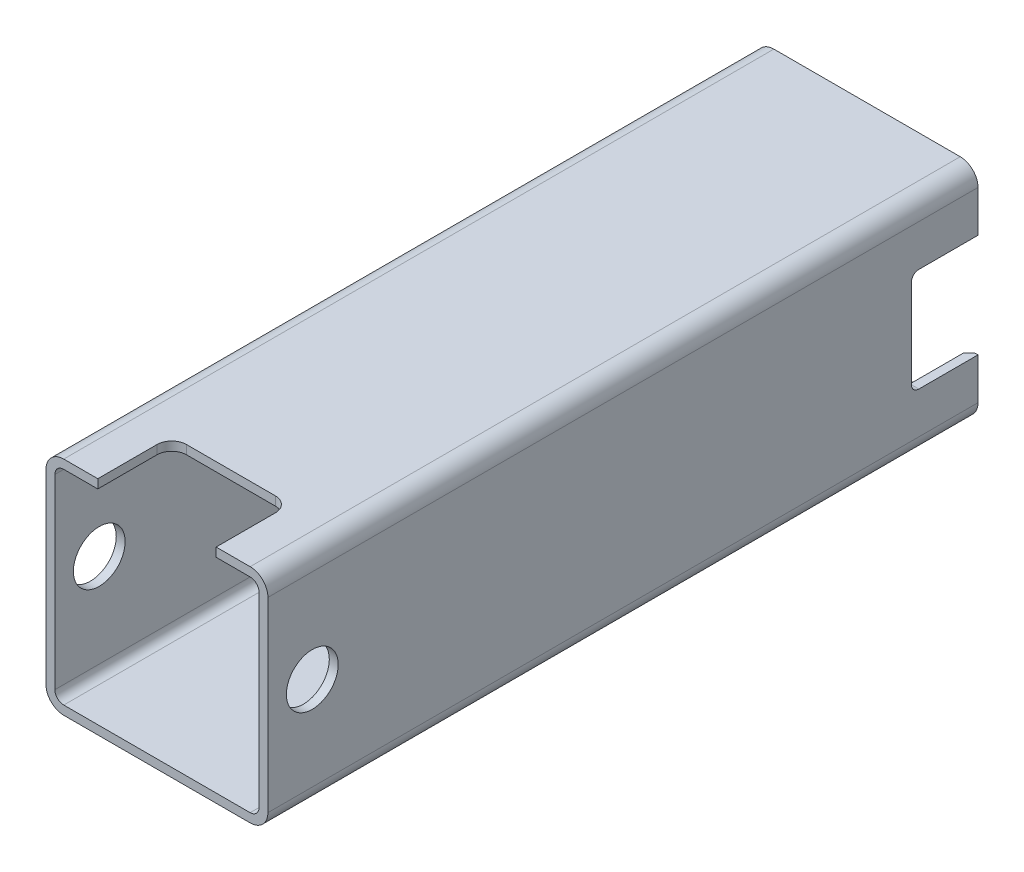
SolidWorks part; units mm, degrees
material "Q235A"
ref_plane "Plane1" through (0, 0, 0) normal (0, 0, 1) x (1, 0, 0)
ref_plane "Plane2" through (0, 0, 0) normal (0, 1, 0) x (1, 0, 0)
ref_plane "Plane3" through (0, 0, 0) normal (1, 0, 0) x (0, 0, -1)
sketch "Sketch1" plane through (0, 0, 0) normal (0, 0, 1) x (1, 0, 0)
  line L0 (-63, -69) -> (63, -69)
  line L1 (-69, -63) -> (-69, 63)
  line L2 (63, 69) -> (-63, 69)
  line L3 (69, 63) -> (69, -63)
  line L4 (-63, -75) -> (63, -75)
  line L5 (-75, -63) -> (-75, 63)
  line L6 (63, 75) -> (-63, 75)
  line L7 (75, 63) -> (75, -63)
  arc A0 (75, 63) -> (63, 75) centre (63, 63) ccw
  arc A1 (63, -75) -> (75, -63) centre (63, -63) ccw
  arc A2 (-75, -63) -> (-63, -75) centre (-63, -63) ccw
  arc A3 (-63, 75) -> (-75, 63) centre (-63, 63) ccw
  arc A4 (-63, 69) -> (-69, 63) centre (-63, 63) ccw
  arc A5 (69, 63) -> (63, 69) centre (63, 63) ccw
  arc A6 (63, -69) -> (69, -63) centre (63, -63) ccw
  arc A7 (-69, -63) -> (-63, -69) centre (-63, -63) ccw
  point P0 (-75, 0)
  point P1 (75, 0)
  point P2 (0, 75)
  point P3 (0, -75)
  point P4 (0, 0)
  point P5 (-75, -75)
  point P6 (75, -75)
  point P7 (75, 75)
  point P8 (-75, 75)
extrude "Boss-Extrude1" add sketch "Sketch1" along normal mid plane 480
sketch "草图1" plane through (0, 0, 0) normal (0, 1, 0) x (1, 0, 0)
  line L0 (63, -240) -> (-63, -240) construction
  line L1 (40, -290) -> (-40, -290)
  line L2 (40, -290) -> (40, -200)
  line L3 (30, -190) -> (-30, -190)
  line L4 (-40, -290) -> (-40, -200)
  line L5 (40, -290) -> (-40, -190) construction
  line L6 (40, -190) -> (-40, -290) construction
  arc A0 (-30, -190) -> (-40, -200) centre (-30, -200) ccw
  arc A1 (40, -200) -> (30, -190) centre (30, -200) ccw
  point P0 (0, -240)
  dimension "D3" = 10
  dimension "D1" = 100
  dimension "D2" = 80
extrude "Cut-Extrude1" cut sketch "草图1" along normal through all
sketch "Sketch2" plane through (0, 0, 0) normal (1, 0, 0) x (0, 0, -1)
  line L0 (240, 63) -> (240, -63) construction
  line L1 (200, 35) -> (285, 35)
  line L2 (195, 30) -> (195, -30)
  line L3 (200, -35) -> (285, -35)
  line L4 (285, 35) -> (285, -35)
  line L5 (195, 35) -> (285, -35) construction
  line L6 (195, -35) -> (285, 35) construction
  line L7 (-240, 63) -> (-240, -63) construction
  arc A0 (195, -30) -> (200, -35) centre (200, -30) ccw
  arc A1 (200, 35) -> (195, 30) centre (200, 30) ccw
  circle A2 centre (-210, 0) radius 17.5
  point P0 (240, 0)
  dimension "D3" = 5
  dimension "D4" = 35
  dimension "D5" = 30
  dimension "D1" = 70
  dimension "D2" = 90
extrude "Cut-Extrude2" cut sketch "Sketch2" against normal through all both and the other way through all
chamfer "Chamfer1" distance 4 angle 45 10 edges at (69, 49, -240) (67.2426, 67.2426, -240) (0, 69, -240) (-67.2426, 67.2426, -240) (-69, 49, -240) (69, -49, -240) (67.2426, -67.2426, -240) (0, -69, -240) (-67.2426, -67.2426, -240) (-69, -49, -240)
